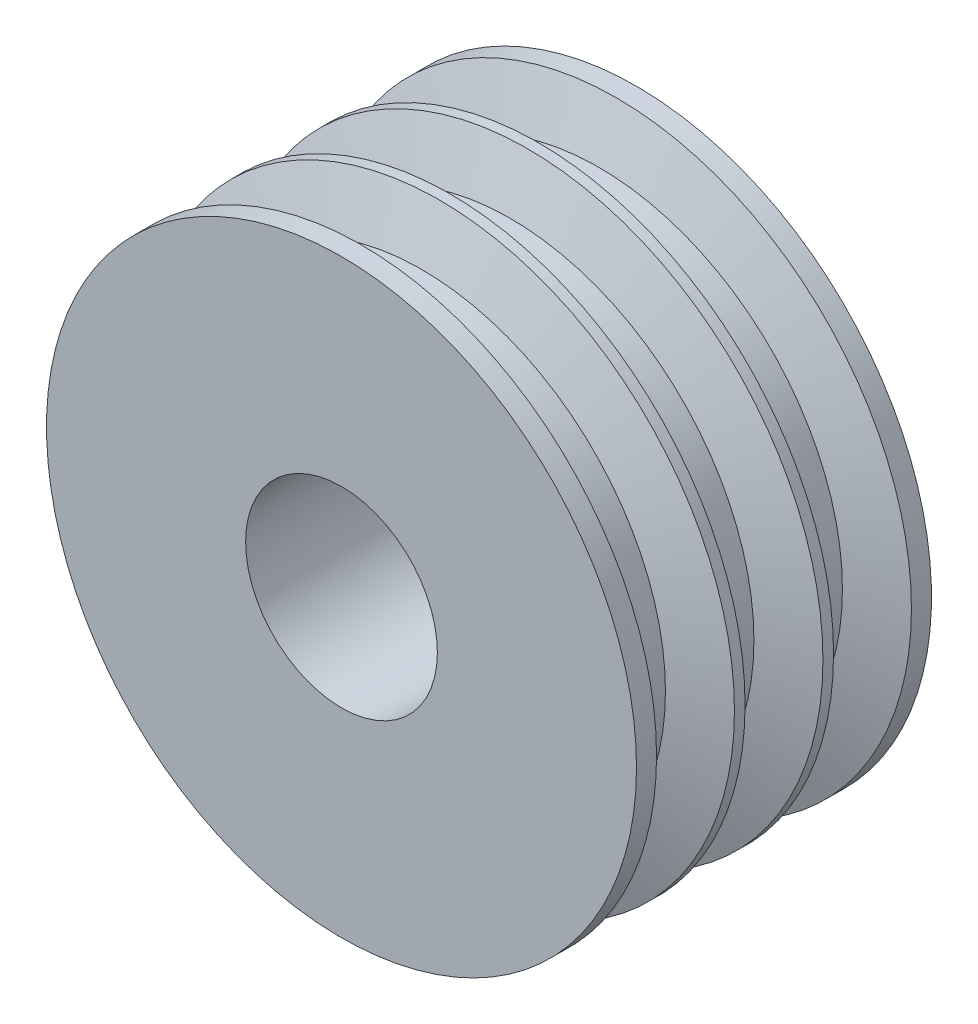
from build123d import *

# Parameters (mm, degrees)
SKETCH1_R           = 50
BOSS_EXTRUDE1_DEPTH = 40
SKETCH2_R           = 16.25
CUT_EXTRUDE1_DEPTH  = 150
SKETCH10_R          = 100
CUT_EXTRUDE5_DEPTH  = 20
SKETCH11_R          = 30
SKETCH11_R_2        = 16.25
BOSS_EXTRUDE2_DEPTH = 20
SKETCH12_R          = 130
CUT_EXTRUDE7_DEPTH  = 30


with BuildPart() as part:
    # Sketch1 → Boss-Extrude1 (new, symmetric)
    with BuildSketch(Plane.XY):
        Circle(SKETCH1_R)
    extrude(amount=BOSS_EXTRUDE1_DEPTH, both=True)

    # Sketch2 → Cut-Extrude1 (cut)
    with BuildSketch(Plane.XY.offset(40)):
        Circle(SKETCH2_R)
    extrude(amount=-CUT_EXTRUDE1_DEPTH, mode=Mode.SUBTRACT)

    # Sketch4 → Cut-Revolve1 (revolve, cut)
    with BuildSketch(Plane(origin=(0, 0, 0), x_dir=(0, 0, -1), z_dir=(1, 0, 0)), mode=Mode.PRIVATE) as cut_revolve1_sk:
        Polygon((-40, 50), (-36.6, 50), (-33.604349764, 41.3), (-26.395650236, 41.3), (-23.4, 50), (-21.6, 50), (-18.604349764, 41.3), (-11.395650236, 41.3), (-8.4, 50), (-6.6, 50), (-3.604349764, 41.3), (3.604349764, 41.3), (6.6, 50), (10, 50), (10, 161.050459045), (-40, 161.050459045), align=None)
    revolve(cut_revolve1_sk.sketch.rotate(Axis((0, 0, 0), (0, 0, -1)), 90), axis=Axis((0, 0, 0), (0, 0, -1)), mode=Mode.SUBTRACT)

    # Sketch10 → Cut-Extrude5 (cut)
    with BuildSketch(Plane(origin=(0, 0, -40), x_dir=(-1, 0, 0), z_dir=(0, 0, -1))):
        Circle(SKETCH10_R)
    extrude(amount=-CUT_EXTRUDE5_DEPTH, mode=Mode.SUBTRACT)

    # Sketch11 → Boss-Extrude2 (add)
    with BuildSketch(Plane(origin=(0, 0, -20), x_dir=(-1, 0, 0), z_dir=(0, 0, -1))):
        Circle(SKETCH11_R)
        with Locations(Location((0, 0, 0), (0, 0, 180))):
            Circle(SKETCH11_R_2, mode=Mode.SUBTRACT)
    extrude(amount=BOSS_EXTRUDE2_DEPTH)

    # Sketch12 → Cut-Extrude7 (cut)
    with BuildSketch(Plane(origin=(0, 0, -40), x_dir=(-1, 0, 0), z_dir=(0, 0, -1))):
        Circle(SKETCH12_R)
    extrude(amount=-CUT_EXTRUDE7_DEPTH, mode=Mode.SUBTRACT)


solid = part.part
